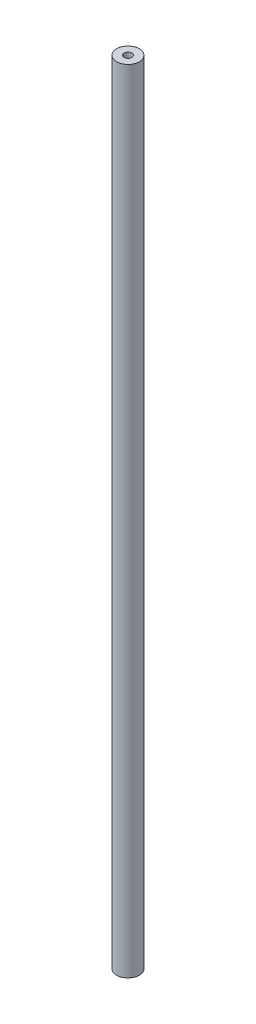
SolidWorks part; units mm, degrees
ref_plane "Front Plane" through (0, 0, 0) normal (0, 0, 1) x (1, 0, 0)
ref_plane "Top Plane" through (0, 0, 0) normal (0, 1, 0) x (1, 0, 0)
ref_plane "Right Plane" through (0, 0, 0) normal (1, 0, 0) x (0, 0, -1)
sketch "Sketch1" plane through (0, 0, 0) normal (0, 1, 0) x (1, 0, 0)
  circle A0 centre (0, 0) radius 10
  dimension "D1" = 20
extrude "Boss-Extrude1" add sketch "Sketch1" along normal blind 700
hole_wizard "M8 Tapped Hole1" positions "Sketch2" profile "Sketch3" tap size "M8" standard "GB"
sketch "Sketch2" plane through (0, 700, 0) normal (0, 1, 0) x (1, 0, 0)
  circle A0 centre (0, 0) radius 10 construction
  point P0 (0, 0)
  point P3 (0, 0)
sketch "Sketch3" plane through (0, 700, 0) normal (1, 0, 0) x (0, 0, 1)
  line L0 (0, 0) -> (0, 21.7929)
  line L1 (0, 21.7929) -> (3.4, 19.75)
  line L2 (3.4, 19.75) -> (3.4, 0)
  line L5 (3.4, 0) -> (0, 0)
  line L10 (0, 21.7929) -> (-3.4, 19.75) construction
  line L11 (0, -6.35) -> (0, 107.95) construction
  dimension "螺纹孔钻头直径" = 6.8
  dimension "螺纹孔钻头深度" = 19.75
  dimension "导头角度" = 118
cosmetic thread "Cosmetic Thread1" parameters "D1"=16, "D2"=8
hole_wizard "M8 Tapped Hole2" positions "Sketch4" profile "Sketch5" tap size "M8" standard "GB"
sketch "Sketch4" plane through (0, 0, 0) normal (0, -1, 0) x (-1, 0, 0)
  point P0 (0, 0)
sketch "Sketch5" plane through (0, 0, 0) normal (1, 0, 0) x (0, 0, -1)
  line L0 (0, 0) -> (0, 21.7929)
  line L1 (0, 21.7929) -> (3.4, 19.75)
  line L2 (3.4, 19.75) -> (3.4, 0)
  line L5 (3.4, 0) -> (0, 0)
  line L10 (0, 21.7929) -> (-3.4, 19.75) construction
  line L11 (0, -6.35) -> (0, 107.95) construction
  dimension "螺纹孔钻头直径" = 6.8
  dimension "螺纹孔钻头深度" = 19.75
  dimension "导头角度" = 118
cosmetic thread "Cosmetic Thread2" parameters "D1"=16, "D2"=8
